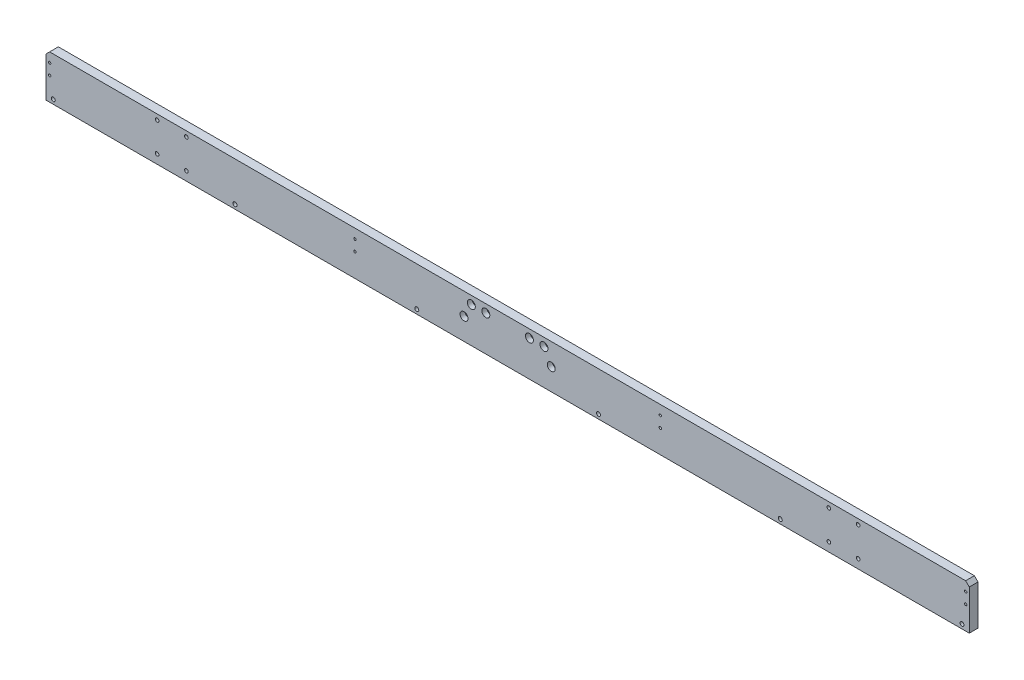
from build123d import *

# Parameters (mm, degrees)
SKETCH_1_W                = 1270
SKETCH_1_H                = 60
EXTRUDE_1_DEPTH           = 12
CHAMFER_1_SIZE            = 5
HOLE_WIZARD_1_D           = 5.5
HOLE_WIZARD_1_CBORE_D     = 10
HOLE_WIZARD_1_CBORE_DEPTH = 5.7
HOLE_WIZARD_M6_1_D        = 5
HOLE_WIZARD_M4_1_D        = 3.3
HOLE_WIZARD_2_D           = 6.6
HOLE_WIZARD_2_CBORE_D     = 11
HOLE_WIZARD_2_CBORE_DEPTH = 6.8


with BuildPart() as part:
    # 草图1 → 凸台-拉伸1 (new body)
    with BuildSketch(Plane.XY):
        Rectangle(SKETCH_1_W, SKETCH_1_H)
    extrude(amount=EXTRUDE_1_DEPTH)

    # 倒角1
    chamfer_1_edges = [part.edges().sort_by_distance(p)[0] for p in [
        (-635, 30, 6),
        (635, 30, 6),
    ]]
    chamfer(chamfer_1_edges, length=CHAMFER_1_SIZE)

    # 打孔尺寸(%根据)内六角圆柱头螺钉的类型1 (through all)
    with Locations(Plane(origin=(0, 0, 0), x_dir=(-1, 0, 0), z_dir=(0, 0, -1))):
        with Locations((-625, -24), (-375, -24), (-125, -24), (125, -24), (375, -24), (625, -24)):
            CounterBoreHole(HOLE_WIZARD_1_D / 2, HOLE_WIZARD_1_CBORE_D / 2, HOLE_WIZARD_1_CBORE_DEPTH)

    # M6 螺纹孔1 (through all)
    with Locations(Plane(origin=(0, 0, 0), x_dir=(-1, 0, 0), z_dir=(0, 0, -1))):
        with Locations((-482.152543264, 22.652543264), (-441.847456736, 22.652543264), (-441.847456736, -17.652543264), (-482.152543264, -17.652543264), (482.152543264, -17.652543264), (441.847456736, -17.652543264), (441.847456736, 22.652543264), (482.152543264, 22.652543264)):
            Hole(HOLE_WIZARD_M6_1_D / 2)

    # M4 螺纹孔1 (through all)
    with Locations(Plane.XY.offset(12)):
        with Locations((-630, 17), (-630, 2), (630, 2), (630, 17), (-210, 17), (-210, 2), (210, 2), (210, 17)):
            Hole(HOLE_WIZARD_M4_1_D / 2)

    # 打孔尺寸(%根据)内六角圆柱头螺钉的类型2 (through all)
    with Locations(Plane.XY.offset(12)):
        with Locations((-60, 0), (-50, 19), (-30, 19), (30, 19), (50, 19), (60, 0)):
            CounterBoreHole(HOLE_WIZARD_2_D / 2, HOLE_WIZARD_2_CBORE_D / 2, HOLE_WIZARD_2_CBORE_DEPTH)


solid = part.part
